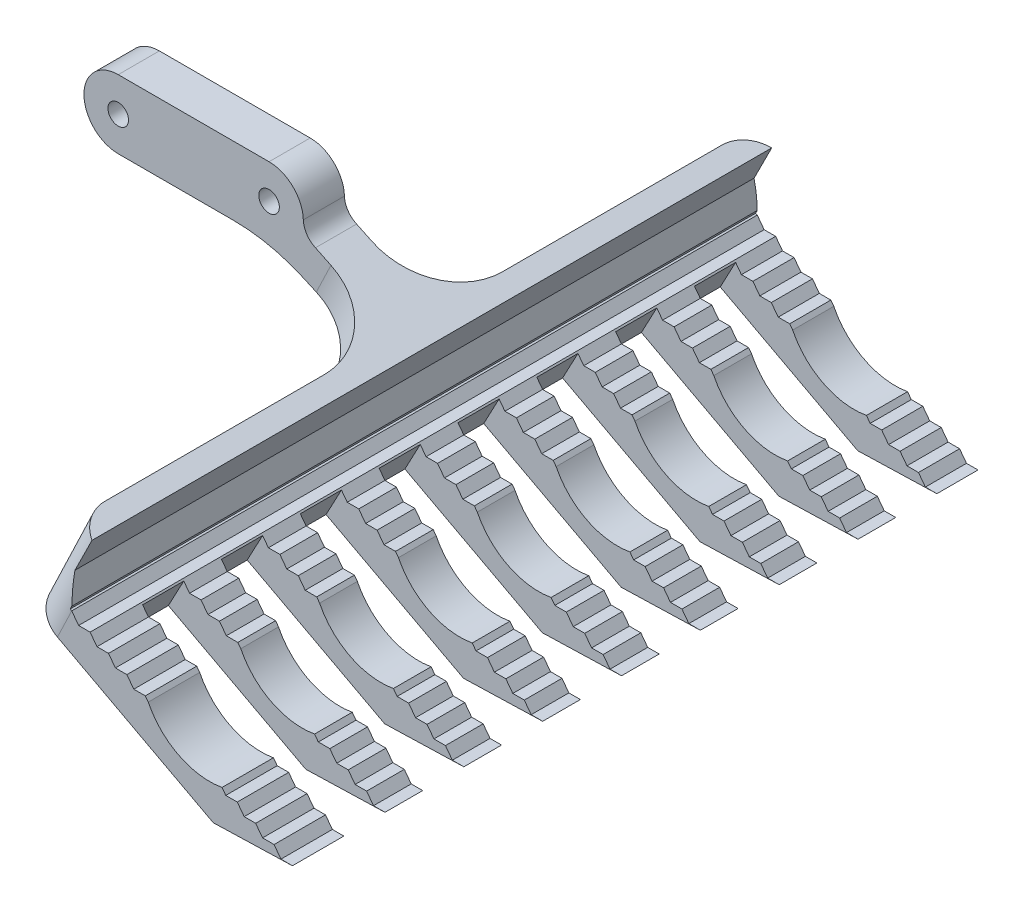
SolidWorks part; units mm, degrees
material "1.0503 (C45)"
ref_plane "Front Plane" through (0, 0, 0) normal (0, 0, 1) x (1, 0, 0)
ref_plane "Top Plane" through (0, 0, 0) normal (0, 1, 0) x (1, 0, 0)
ref_plane "Right Plane" through (0, 0, 0) normal (1, 0, 0) x (0, 0, -1)
ref_plane "Plane1" through (0, 0, 6) normal (0, 0, 1) x (1, 0, 0)
sketch "Sketch1" plane through (0, 0, 6) normal (0, 0, 1) x (1, 0, 0)
  line L0 (35.197, -5.9165) -> (35.197, -5.3686)
  line L1 (35.197, -5.3686) -> (34.9453, -5.2557)
  line L2 (34.9453, -5.2557) -> (29.0116, -7.527)
  line L3 (29.0116, -7.527) -> (17.7688, -2.4866)
  line L4 (11, 5) -> (-11, 5)
  line L5 (-11, -5) -> (5.8051, -5)
  line L6 (16.0324, -7.1877) -> (30.6027, -13.7199)
  line L7 (43.1577, -8.9375) -> (42.906, -8.8247)
  line L8 (42.906, -8.8247) -> (42.497, -9.1892)
  line L9 (42.497, -9.1892) -> (42.497, -8.6413)
  line L10 (42.497, -8.6413) -> (41.9935, -8.4156)
  line L11 (41.9935, -8.4156) -> (41.5845, -8.7801)
  line L12 (41.5845, -8.7801) -> (41.5845, -8.2322)
  line L13 (41.5845, -8.2322) -> (41.0811, -8.0065)
  line L14 (41.0811, -8.0065) -> (40.672, -8.3711)
  line L15 (40.672, -8.3711) -> (40.672, -7.8231)
  line L16 (40.672, -7.8231) -> (40.1686, -7.5974)
  line L17 (40.1686, -7.5974) -> (39.7595, -7.962)
  line L18 (39.7595, -7.962) -> (39.7595, -7.414)
  line L19 (39.7595, -7.414) -> (39.2561, -7.1883)
  line L20 (39.2561, -7.1883) -> (38.847, -7.5529)
  line L21 (38.847, -7.5529) -> (38.847, -7.0049)
  line L22 (38.847, -7.0049) -> (38.3436, -6.7792)
  line L23 (38.3436, -6.7792) -> (37.9345, -7.1438)
  line L24 (37.9345, -7.1438) -> (37.9345, -6.5958)
  line L25 (37.9345, -6.5958) -> (37.4311, -6.3701)
  line L26 (37.4311, -6.3701) -> (37.022, -6.7347)
  line L27 (37.022, -6.7347) -> (37.022, -6.1867)
  line L28 (37.022, -6.1867) -> (36.5186, -5.9611)
  line L29 (36.5186, -5.9611) -> (36.1095, -6.3256)
  line L30 (36.1095, -6.3256) -> (36.1095, -5.7776)
  line L31 (36.1095, -5.7776) -> (35.6061, -5.552)
  line L32 (35.6061, -5.552) -> (35.197, -5.9165)
  arc A0 (17.7688, -2.4866) -> (15.9975, 0.1568) centre (18.9961, 0.2508) cw
  arc A1 (15.9975, 0.1568) -> (11, 5) centre (11, 0) ccw
  arc A2 (-11, 5) -> (-11, -5) centre (-11, 0) ccw
  arc A3 (5.8051, -5) -> (16.0324, -7.1877) centre (5.8051, -30) cw
  arc A4 (30.6027, -13.7199) -> (43.1577, -8.9375) centre (34.4891, -5.0512) ccw
  circle A5 centre (-11, 0) radius 1.5
  circle A6 centre (11, 0) radius 1.5
  circle A7 centre (36.5498, -11.4545) radius 1.5
extrude "Boss-Extrude1" add sketch "Sketch1" against normal blind 6
sketch "Sketch6" plane through (0, 0, 6) normal (0, 0, 1) x (1, 0, 0)
  line L0 (17.7688, -2.4866) -> (29.0492, -7.873)
  line L1 (29.0492, -7.873) -> (25.3766, -15.5643)
  line L2 (25.3766, -15.5643) -> (48.3397, -22.9328)
  line L3 (48.3397, -22.9328) -> (43.962, 0.8987)
  line L4 (43.962, 0.8987) -> (17.7688, -2.4866)
extrude "Cut-Extrude1" cut sketch "Sketch6" against normal blind 10
sketch "Sketch7" plane through (0, 0, 6) normal (0, 0, 1) x (1, 0, 0)
  line L3 (29.0492, -7.873) -> (27.0235, -12.1152)
  line L4 (0, 0) -> (-23.2645, -48.7217) construction
  line L5 (22.7146, -21.1393) -> (58.0325, -39.9181)
  line L6 (58.0325, -39.9181) -> (69.4616, -39.2577)
  line L7 (69.4616, -39.2577) -> (28.98, -19.0169)
  line L8 (24.7402, -16.897) -> (22.7146, -21.1393)
  line L9 (27.0235, -12.1152) -> (24.7402, -16.897)
  line L10 (29.0492, -7.873) -> (33.4913, -9.9941)
  line L11 (33.4913, -9.9941) -> (28.98, -19.0169)
  dimension "D1" = 18.7789
  dimension "D2" = 4.9226
  dimension "D3" = 10.0878
  dimension "D4" = 40
  dimension "D5" = 11.4291
extrude "Boss-Extrude2" add sketch "Sketch7" along normal mid plane 100 from offset 3
fillet "Fillet1" radius 10 2 edges at (28.0364, -9.9941, 0) (28.0364, -9.9941, 6)
fillet "Fillet2" radius 5 2 edges at (25.8819, -14.5061, -47) (25.8819, -14.5061, 53)
sketch "Sketch8" plane through (0, 0, 53) normal (0, 0, 1) x (1, 0, 0)
  line L0 (34.5283, -11.4511) -> (33.5221, -10.1095)
  line L1 (34.5283, -11.4511) -> (36.2053, -11.4511)
  line L2 (37.2116, -12.7927) -> (36.2053, -11.4511)
  line L3 (37.2116, -12.7927) -> (38.8886, -12.7927)
  line L4 (39.8949, -14.1344) -> (38.8886, -12.7927)
  line L5 (39.8949, -14.1344) -> (41.5719, -14.1344)
  line L6 (42.5781, -15.476) -> (41.5719, -14.1344)
  line L7 (42.5781, -15.476) -> (44.2552, -15.476)
  line L8 (45.2614, -16.8177) -> (44.2552, -15.476)
  line L9 (45.2614, -16.8177) -> (46.9385, -16.8177)
  line L10 (47.9447, -18.1593) -> (46.9385, -16.8177)
  line L11 (47.9447, -18.1593) -> (49.6217, -18.1593)
  line L12 (50.628, -19.501) -> (49.6217, -18.1593)
  line L13 (50.628, -19.501) -> (52.305, -19.501)
  line L14 (53.3113, -20.8426) -> (52.305, -19.501)
  line L15 (53.3113, -20.8426) -> (54.9883, -20.8426)
  line L16 (55.9945, -22.1842) -> (54.9883, -20.8426)
  line L17 (55.9945, -22.1842) -> (57.6716, -22.1842)
  line L18 (58.6778, -23.5259) -> (57.6716, -22.1842)
  line L19 (58.6778, -23.5259) -> (60.3549, -23.5259)
  line L20 (61.3611, -24.8675) -> (60.3549, -23.5259)
  line L21 (61.3611, -24.8675) -> (63.0382, -24.8675)
  line L22 (64.0444, -26.2092) -> (63.0382, -24.8675)
  line L23 (64.0444, -26.2092) -> (65.7214, -26.2092)
  line L24 (66.7277, -27.5508) -> (65.7214, -26.2092)
  line L25 (66.7277, -27.5508) -> (68.4047, -27.5508)
  line L26 (69.4109, -28.8925) -> (68.4047, -27.5508)
  line L27 (69.4109, -28.8925) -> (71.088, -28.8925)
  line L28 (71.088, -28.8925) -> (72.1236, -25.3238)
  line L29 (72.1236, -25.3238) -> (33.5221, -5.2127)
  line L30 (33.5221, -5.2127) -> (33.5221, -10.1095)
  line L31 (43.6357, -27.1833) -> (45.3128, -27.1833)
  line L32 (46.319, -28.525) -> (45.3128, -27.1833)
  line L33 (46.319, -28.525) -> (47.9961, -28.525)
  line L34 (49.0023, -29.8666) -> (47.9961, -28.525)
  line L35 (49.0023, -29.8666) -> (50.6794, -29.8666)
  line L36 (51.6856, -31.2083) -> (50.6794, -29.8666)
  line L37 (51.6856, -31.2083) -> (53.3626, -31.2083)
  line L38 (54.3689, -32.5499) -> (53.3626, -31.2083)
  line L39 (54.3689, -32.5499) -> (56.0459, -32.5499)
  line L40 (57.0521, -33.8915) -> (56.0459, -32.5499)
  line L41 (57.0521, -33.8915) -> (58.7292, -33.8915)
  line L42 (59.7354, -35.2332) -> (58.7292, -33.8915)
  line L43 (59.7354, -35.2332) -> (61.4125, -35.2332)
  line L44 (62.4187, -36.5748) -> (61.4125, -35.2332)
  line L45 (62.4187, -36.5748) -> (64.0958, -36.5748)
  line L46 (65.102, -37.9165) -> (64.0958, -36.5748)
  line L47 (65.102, -37.9165) -> (66.779, -37.9165)
  line L48 (66.779, -37.9165) -> (67.8146, -34.3478)
  line L49 (67.8146, -34.3478) -> (29.2131, -14.2368)
  line L50 (40.9525, -25.8417) -> (39.9462, -24.5)
  line L51 (38.2692, -24.5) -> (39.9462, -24.5)
  line L52 (38.2692, -24.5) -> (37.263, -23.1584)
  line L53 (35.5859, -23.1584) -> (37.263, -23.1584)
  line L54 (35.5859, -23.1584) -> (34.5797, -21.8168)
  line L55 (32.9026, -21.8168) -> (34.5797, -21.8168)
  line L56 (32.9026, -21.8168) -> (31.8964, -20.4751)
  line L57 (30.2193, -20.4751) -> (31.8964, -20.4751)
  line L58 (30.2193, -20.4751) -> (29.2131, -19.1335)
  line L59 (29.2131, -14.2368) -> (29.2131, -19.1335)
  line L60 (43.6357, -27.1833) -> (42.6295, -25.8417)
  line L61 (42.6295, -25.8417) -> (40.9525, -25.8417)
  dimension "D1" = 2
extrude "Cut-Extrude2" cut sketch "Sketch8" against normal blind 100
ref_plane "Plane2" through (0.9341, 1.7568, 0) normal (-0.4695, -0.8829, 0) x (-0.8829, 0.4695, 0)
sketch "Sketch13" plane through (0.9341, 1.7568, 0) normal (-0.4695, -0.8829, 0) x (-0.8829, 0.4695, 0)
  line L0 (-38.0201, 23.5) -> (-83.0201, 23.5)
  line L1 (-38.0201, 41) -> (-83.0201, 41)
  line L2 (-83.0201, 41) -> (-83.0201, 35)
  line L3 (-38.0201, 41) -> (-38.0201, 35)
  line L4 (-38.0201, 35) -> (-83.0201, 35)
  line L5 (-38.0201, 29.5) -> (-38.0201, 23.5)
  line L6 (-38.0201, 29.5) -> (-83.0201, 29.5)
  line L7 (-83.0201, 29.5) -> (-83.0201, 23.5)
  line L8 (-38.0201, 12) -> (-83.0201, 12)
  line L9 (-38.0201, 18) -> (-38.0201, 12)
  line L10 (-38.0201, 18) -> (-83.0201, 18)
  line L11 (-83.0201, 18) -> (-83.0201, 12)
  line L12 (-38.0201, 0.5) -> (-83.0201, 0.5)
  line L13 (-38.0201, 6.5) -> (-38.0201, 0.5)
  line L14 (-38.0201, 6.5) -> (-83.0201, 6.5)
  line L15 (-83.0201, 6.5) -> (-83.0201, 0.5)
  line L16 (-38.0201, -11) -> (-83.0201, -11)
  line L17 (-38.0201, -5) -> (-38.0201, -11)
  line L18 (-38.0201, -5) -> (-83.0201, -5)
  line L19 (-83.0201, -5) -> (-83.0201, -11)
  line L20 (-38.0201, -22.5) -> (-83.0201, -22.5)
  line L21 (-38.0201, -16.5) -> (-38.0201, -22.5)
  line L22 (-38.0201, -16.5) -> (-83.0201, -16.5)
  line L23 (-83.0201, -16.5) -> (-83.0201, -22.5)
  line L24 (-38.0201, -34) -> (-83.0201, -34)
  line L25 (-38.0201, -28) -> (-38.0201, -34)
  line L26 (-38.0201, -28) -> (-83.0201, -28)
  line L27 (-83.0201, -28) -> (-83.0201, -34)
  line L28 (-38.0201, -45.5) -> (-83.0201, -45.5)
  line L29 (-38.0201, -39.5) -> (-38.0201, -45.5)
  line L30 (-38.0201, -39.5) -> (-83.0201, -39.5)
  line L31 (-83.0201, -39.5) -> (-83.0201, -45.5)
sketch "Sketch10" plane through (0, 0, -47) normal (0, 0, -1) x (-1, 0, 0)
  circle A0 centre (-49.3399, -20.6407) radius 10
  dimension "D1" = 20
extrude "Cut-Extrude4" cut sketch "Sketch10" against normal through all
extrude "Cut-Extrude5" cut sketch "Sketch13" against normal through all both and the other way through all
sketch "Sketch11" plane through (0, 0, 0) normal (0, 0, 1) x (1, 0, 0)
  line L0 (29.2131, -14.2368) -> (31.7501, -9.1627)
  line L1 (33.4913, -9.9941) -> (29.0492, -7.873) construction
  line L2 (31.7501, -9.1627) -> (33.4913, -9.9941)
  line L3 (33.4913, -9.9941) -> (30.9243, -15.1283)
  line L4 (30.9243, -15.1283) -> (29.2131, -14.2368)
extrude "Cut-Extrude6" cut sketch "Sketch11" against normal through all both and the other way through all
sketch "Sketch15" plane through (0, 0, 53) normal (0, 0, 1) x (1, 0, 0)
  line L0 (49.8605, -35.573) -> (61.4125, -35.2332)
  line L1 (27.1335, -23.4888) -> (58.0325, -39.9181) construction
  line L2 (61.4125, -35.2332) -> (69.4616, -39.2577)
  line L3 (69.4616, -39.2577) -> (58.0325, -39.9181)
  line L4 (58.0325, -39.9181) -> (69.4616, -39.2577) construction
  line L5 (58.0325, -39.9181) -> (49.8605, -35.573)
extrude "Cut-Extrude7" cut sketch "Sketch15" against normal through all
